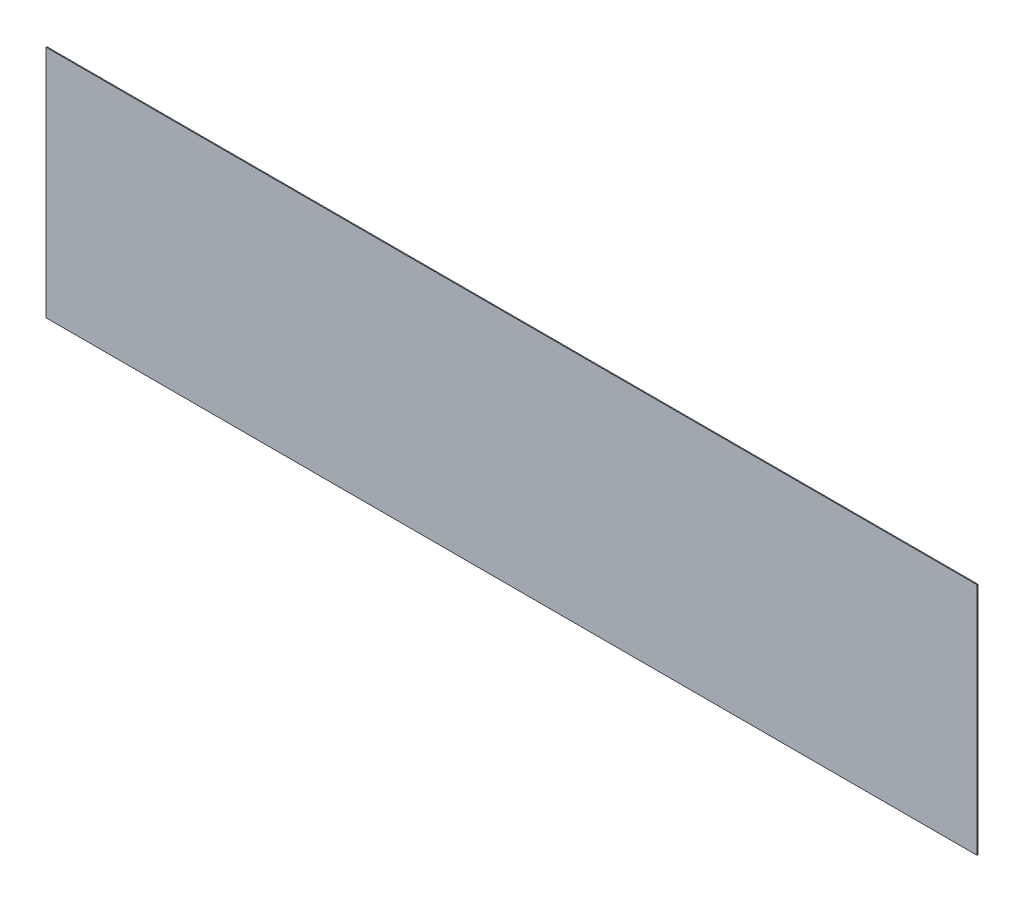
SolidWorks part; units mm, degrees
material "普通碳钢"
ref_plane "Front Plane" through (0, 0, 0) normal (0, 0, 1) x (1, 0, 0)
ref_plane "Top Plane" through (0, 0, 0) normal (0, 1, 0) x (1, 0, 0)
ref_plane "Right Plane" through (0, 0, 0) normal (1, 0, 0) x (0, 0, -1)
sketch "Sketch1" plane through (0, 0, 0) normal (0, 0, 1) x (1, 0, 0)
  line L5 (0, 0) -> (6000, 0)
  line L6 (0, 0) -> (0, 1510)
  line L7 (0, 1510) -> (6000, 1510)
  line L8 (6000, 0) -> (6000, 1510)
  dimension "D2" = 1510
  dimension "D3" = 6000
extrude "Boss-Extrude1" add sketch "Sketch1" along normal blind 6
